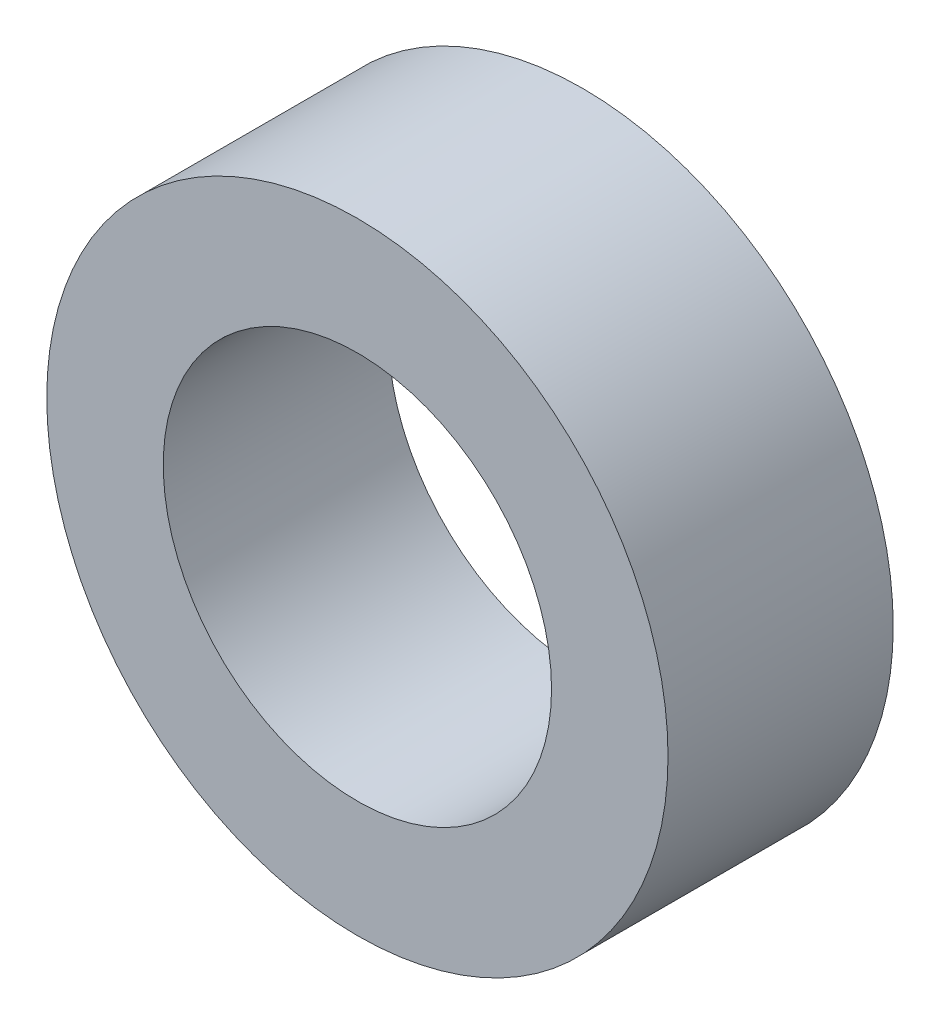
from build123d import *

# Parameters (mm, degrees)
SKETCH1_R           = 4
SKETCH1_R_2         = 2.5
BOSS_EXTRUDE1_DEPTH = 2.9


with BuildPart() as part:
    # Sketch1 → Boss-Extrude1 (new body)
    with BuildSketch(Plane.XY):
        Circle(SKETCH1_R)
        Circle(SKETCH1_R_2, mode=Mode.SUBTRACT)
    extrude(amount=BOSS_EXTRUDE1_DEPTH)


solid = part.part
